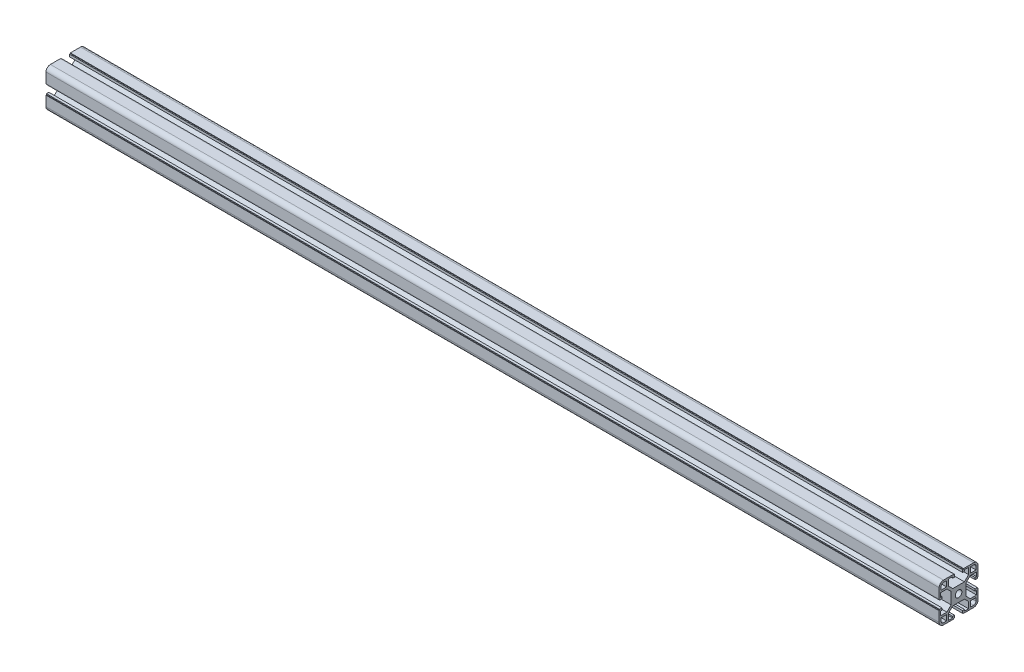
SolidWorks part; units mm, degrees
ref_plane "Front Plane" through (0, 0, 0) normal (0, 0, 1) x (1, 0, 0)
ref_plane "Top Plane" through (0, 0, 0) normal (0, 1, 0) x (1, 0, 0)
ref_plane "Right Plane" through (0, 0, 0) normal (1, 0, 0) x (0, 0, -1)
sketch "草图1" plane through (0, 0, 0) normal (0, 0, 1) x (1, 0, 0)
  line L0 (0, 0) -> (920, 0)
  dimension "D1" = 920
other "Aluminum profile 40 X 40B X R4.5(1)"
ref_plane "Plane1" through (0, 0, 0) normal (1, 0, 0) x (0, 1, 0)
sketch "Sketch1" plane through (0, 0, 0) normal (1, 0, 0) x (0, 1, 0)
  line L0 (-5.1, 20) -> (-5.1, 19.5)
  line L1 (-5.1, 19.5) -> (-4.1, 19.5)
  line L2 (-4.1, 19.5) -> (-4.1, 17)
  line L3 (-6.1, 18.5) -> (-10.3, 18.5)
  line L4 (-15.5, -20) -> (-5.1, -20)
  line L5 (-20, -15.5) -> (-20, -5.1)
  line L6 (15.5, 20) -> (5.1, 20)
  line L7 (20, 15.5) -> (20, 5.1)
  line L8 (0, 14.8756) -> (0, 0) construction
  line L9 (0, 0) -> (14.1675, 0) construction
  line L10 (-10.3, 18.5) -> (-10.3, 12)
  line L11 (-10.3, 12) -> (-6, 7.7)
  line L12 (-6, 7.7) -> (6, 7.7)
  line L13 (10.3, 12) -> (6, 7.7)
  line L14 (10.3, 18.5) -> (10.3, 12)
  line L15 (6.1, 18.5) -> (10.3, 18.5)
  line L16 (4.1, 19.5) -> (4.1, 17)
  line L17 (5.1, 19.5) -> (4.1, 19.5)
  line L18 (5.1, 20) -> (5.1, 19.5)
  line L19 (-5.1, 20) -> (-15.5, 20)
  line L20 (20, 5.1) -> (19.5, 5.1)
  line L21 (12.3, 18) -> (15.5, 18)
  line L22 (12.3, 18) -> (12.3, 12.3)
  line L23 (12.3, 12.3) -> (18, 12.3)
  line L24 (18, 15.5) -> (18, 12.3)
  line L25 (19.5, 5.1) -> (19.5, 4.1)
  line L26 (19.5, 4.1) -> (17, 4.1)
  line L27 (17, 6.1) -> (17, 4.1)
  line L28 (18.5, 6.1) -> (17, 6.1)
  line L29 (18.5, 6.1) -> (18.5, 10.3)
  line L30 (18.5, 10.3) -> (12, 10.3)
  line L31 (12, 10.3) -> (7.7, 6)
  line L32 (7.7, 6) -> (7.7, -6)
  line L33 (12, -10.3) -> (7.7, -6)
  line L34 (18.5, -10.3) -> (12, -10.3)
  line L35 (18.5, -6.1) -> (18.5, -10.3)
  line L36 (18.5, -6.1) -> (17, -6.1)
  line L37 (17, -4.1) -> (17, -6.1)
  line L38 (19.5, -4.1) -> (17, -4.1)
  line L39 (19.5, -5.1) -> (19.5, -4.1)
  line L40 (20, -5.1) -> (19.5, -5.1)
  line L41 (5.1, -20) -> (5.1, -19.5)
  line L42 (5.1, -19.5) -> (4.1, -19.5)
  line L43 (4.1, -19.5) -> (4.1, -17)
  line L44 (6.1, -17) -> (4.1, -17)
  line L45 (6.1, -18.5) -> (6.1, -17)
  line L46 (6.1, -18.5) -> (10.3, -18.5)
  line L47 (10.3, -18.5) -> (10.3, -12)
  line L48 (10.3, -12) -> (6, -7.7)
  line L49 (6, -7.7) -> (-6, -7.7)
  line L50 (-10.3, -12) -> (-6, -7.7)
  line L51 (-10.3, -18.5) -> (-10.3, -12)
  line L52 (-6.1, -18.5) -> (-10.3, -18.5)
  line L53 (-6.1, -18.5) -> (-6.1, -17)
  line L54 (-4.1, -17) -> (-6.1, -17)
  line L55 (-4.1, -19.5) -> (-4.1, -17)
  line L56 (-5.1, -19.5) -> (-4.1, -19.5)
  line L57 (-5.1, -20) -> (-5.1, -19.5)
  line L58 (-20, -5.1) -> (-19.5, -5.1)
  line L59 (5.1, -20) -> (15.5, -20)
  line L60 (-20, 5.1) -> (-20, 15.5)
  line L61 (-19.5, -5.1) -> (-19.5, -4.1)
  line L62 (-6.1, 18.5) -> (-6.1, 17)
  line L63 (-6.1, 17) -> (-4.1, 17)
  line L64 (6.1, 18.5) -> (6.1, 17)
  line L65 (4.1, 17) -> (6.1, 17)
  line L66 (-19.5, -4.1) -> (-17, -4.1)
  line L67 (-15.5, 18) -> (-12.3, 18)
  line L68 (-18, 15.5) -> (-18, 12.3)
  line L69 (-18, 12.3) -> (-12.3, 12.3)
  line L70 (-12.3, 18) -> (-12.3, 12.3)
  line L71 (-17, -6.1) -> (-17, -4.1)
  line L72 (-18.5, -6.1) -> (-17, -6.1)
  line L73 (-18.5, -6.1) -> (-18.5, -10.3)
  line L74 (-18.5, -10.3) -> (-12, -10.3)
  line L75 (-12, -10.3) -> (-7.7, -6)
  line L76 (-7.7, -6) -> (-7.7, 6)
  line L77 (-12, 10.3) -> (-7.7, 6)
  line L78 (-18.5, 10.3) -> (-12, 10.3)
  line L79 (-18.5, 6.1) -> (-18.5, 10.3)
  line L80 (-18.5, 6.1) -> (-17, 6.1)
  line L81 (-17, 4.1) -> (-17, 6.1)
  line L82 (-19.5, 4.1) -> (-17, 4.1)
  line L83 (-19.5, 5.1) -> (-19.5, 4.1)
  line L84 (-20, 5.1) -> (-19.5, 5.1)
  line L85 (20, -5.1) -> (20, -15.5)
  line L87 (-18, -12.3) -> (-12.3, -12.3)
  line L88 (-18, -12.3) -> (-18, -15.5)
  line L89 (-15.5, -18) -> (-12.3, -18)
  line L90 (-12.3, -12.3) -> (-12.3, -18)
  line L91 (12.3, -12.3) -> (18, -12.3)
  line L92 (12.3, -12.3) -> (12.3, -18)
  line L93 (12.3, -18) -> (15.5, -18)
  line L94 (18, -12.3) -> (18, -15.5)
  circle A0 centre (0, 0) radius 3.4
  arc A1 (-20, 15.5) -> (-15.5, 20) centre (-15.5, 15.5) cw
  arc A2 (20, 15.5) -> (15.5, 20) centre (15.5, 15.5) ccw
  arc A3 (-15.5, -20) -> (-20, -15.5) centre (-15.5, -15.5) cw
  arc A4 (15.5, -20) -> (20, -15.5) centre (15.5, -15.5) ccw
  arc A5 (-15.5, 18) -> (-18, 15.5) centre (-15.5, 15.5) ccw
  arc A6 (18, 15.5) -> (15.5, 18) centre (15.5, 15.5) ccw
  arc A7 (18, -15.5) -> (15.5, -18) centre (15.5, -15.5) cw
  arc A8 (-18, -15.5) -> (-15.5, -18) centre (-15.5, -15.5) ccw
  point P2 (0, 10)
  point P4 (0, 0)
  point P5 (-20, -20)
  point P6 (20, -20)
  point P7 (20, 20)
  point P8 (-20, 20)
  point P36 (-20, 20)
  point P39 (20, 20)
  point P121 (0, 0)
  dimension "D1" = 20.6
  dimension "D2" = 40
  dimension "D3" = 8.2
  dimension "D4" = 10.2
  dimension "D5" = 12.3
  dimension "D6" = 6.8
  dimension "D7" = 4.5
  dimension "D8" = 45
  dimension "D12" = 2
  dimension "D13" = 5.7
  dimension "D14" = 2
  dimension "D18" = 2.5
  dimension "D19" = 2.5
  dimension "D15" = 2.5
  dimension "D9" = 0.5
  dimension "D10" = 1.5
  dimension "D11" = 12
  dimension "D16" = 3
  dimension "D17" = 2
  dimension "D20" = 2
  dimension "D21" = 2
